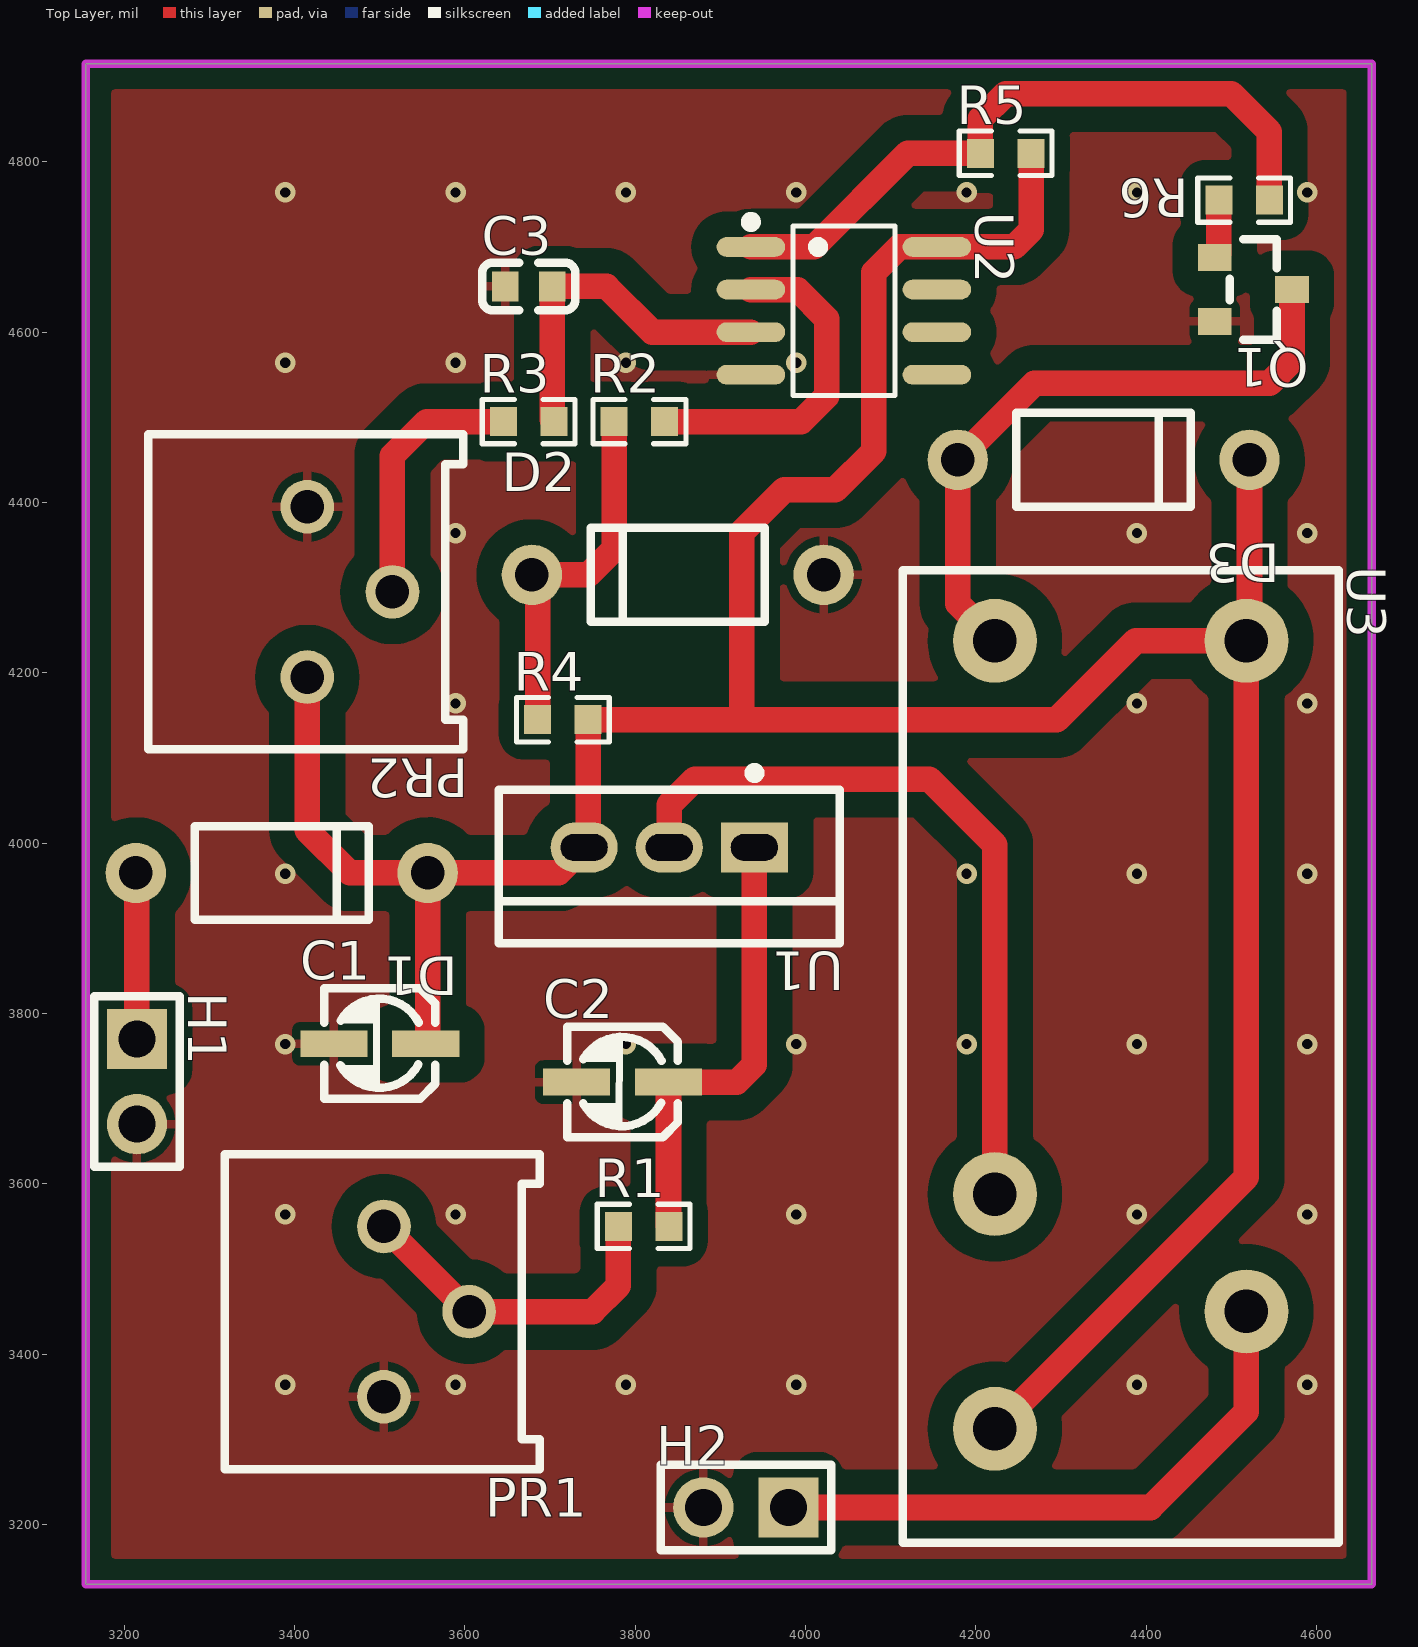
[diagram p0: Top Layer view]
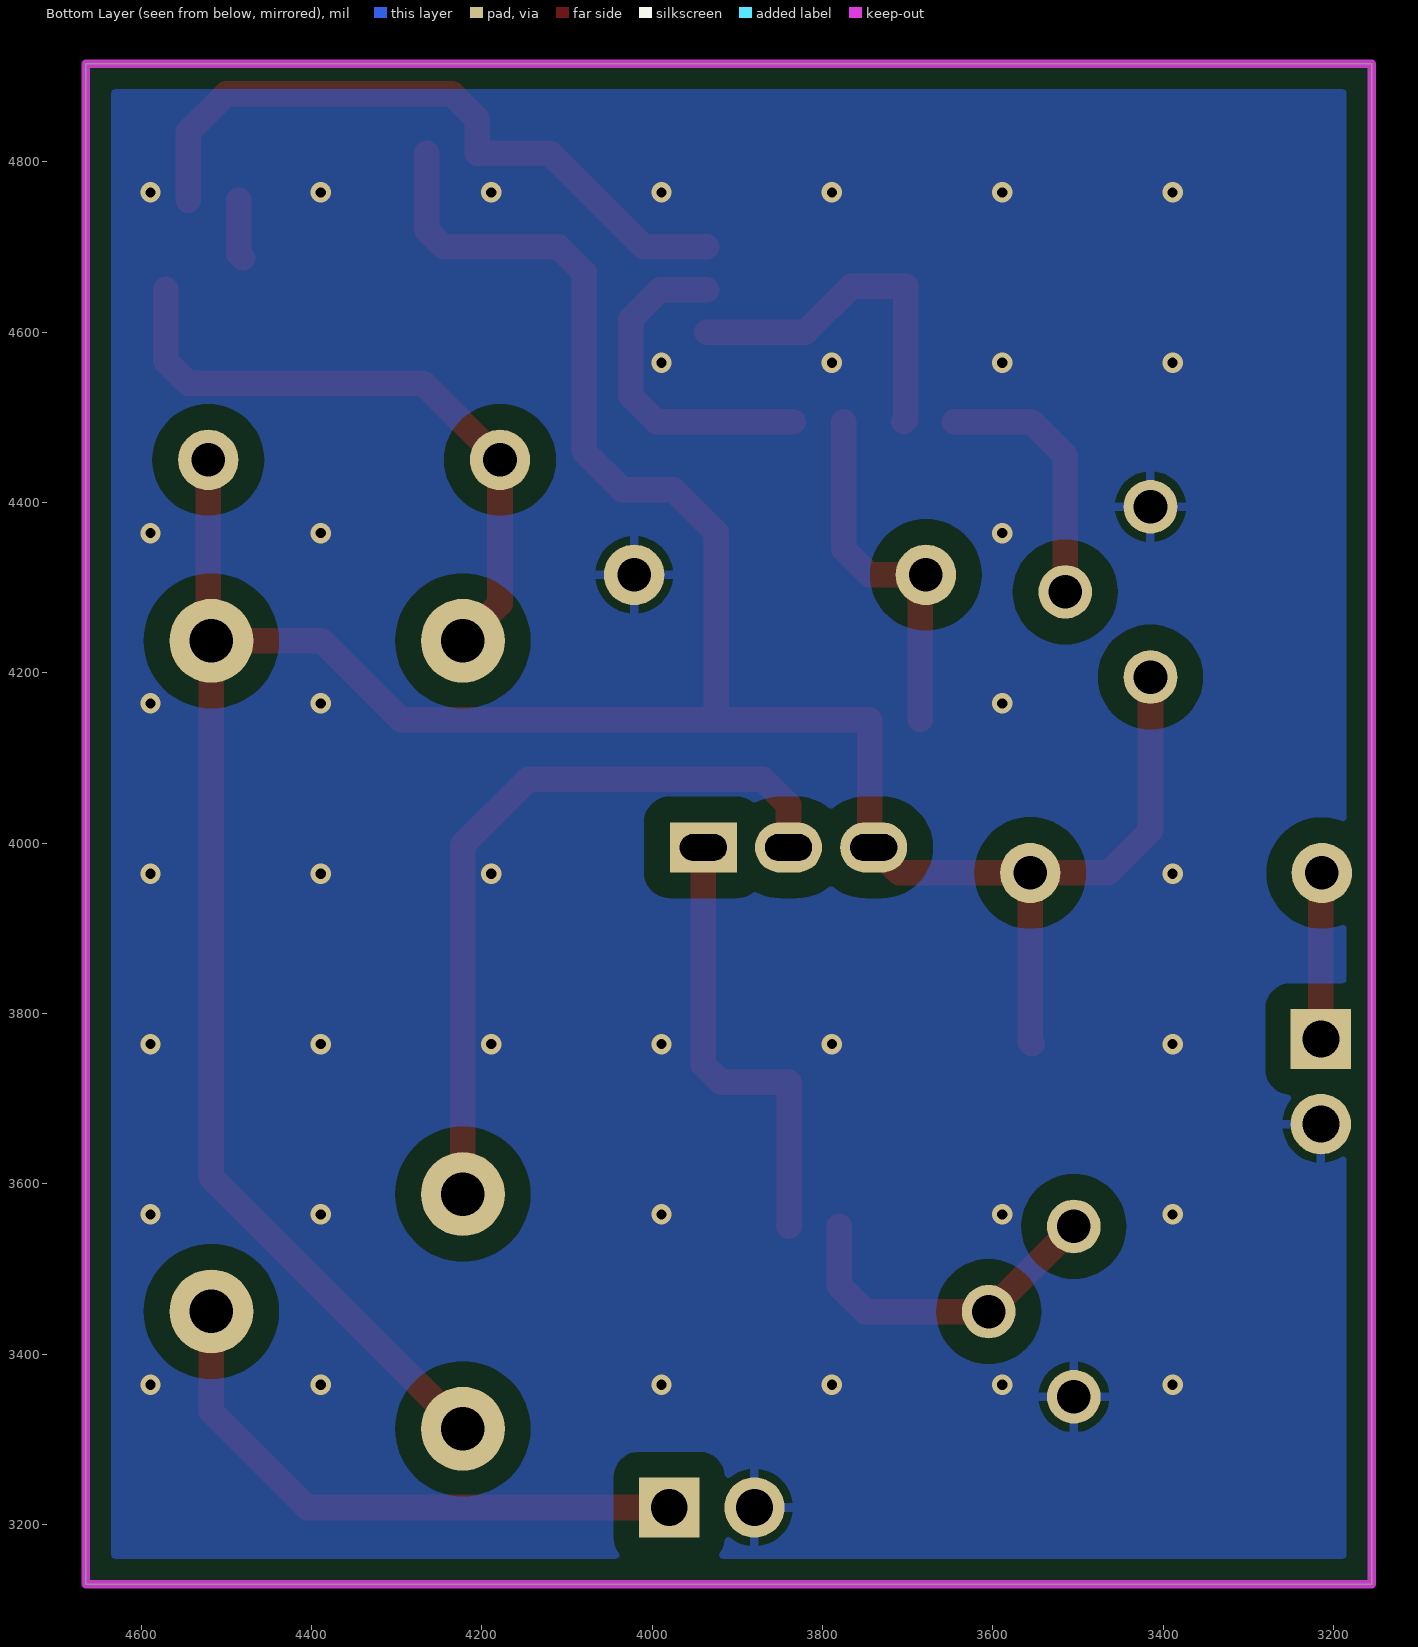
[diagram p1: Bottom Layer view, seen from below]
# Altium PCB MISC52117.pcbdoc
Units mil, origin at the board's own origin, x right, y up, seen from the top; angles counter-clockwise.
Board outline 1510 x 1785 mil, 2 copper layers (Top Layer, Bottom Layer), stack 62.206 mil thick; 20 components, 14 nets, 53 pads, 38 vias.

## Layer stack, top to bottom
Top Solder Mask Layer: solder mask 0.394, Dk 3.3
Top Layer: signal copper 1.379
Dielectric1: surface 59.449, FR4, Dk 4.5
Bottom Layer: signal copper 1.378
Bottom Solder Mask Layer: solder mask 0.394, Dk 3.3

## Board outline
3155,4915 3155,3130 4665,3130 4665,4915

## Design rules (kind name [scope] priority, off if disabled: settings)
BoardOutlineClearance copperThickness2oz_1 [All] p2 off: genericclearance=7.99 ignorepadtopadclearanceinfootprint=FALSE except(0: Arc-SplitContinuation Track-SplitContinuation SMDPad-SplitContinuation THPad-SplitContinuation Via-SplitContinuation Fill-SplitContinuation Region-SplitContinuation Poly-SplitContinuation Text-SplitContinuation Hole-SplitContinuation; 5.98: Arc-CutoutEdge Track-CutoutEdge SMDPad-CutoutEdge THPad-CutoutEdge Via-CutoutEdge Text-CutoutEdge; 6.89: Hole-OutlineEdge Hole-CutoutEdge; 11.81: Arc-OutlineEdge Track-OutlineEdge SMDPad-OutlineEdge THPad-OutlineEdge Via-OutlineEdge Fill-OutlineEdge Region-OutlineEdge Text-OutlineEdge Fill-CutoutEdge Region-CutoutEdge; 30: Poly-OutlineEdge Poly-CutoutEdge)
BoardOutlineClearance Plane_innerPlane_1 [All] p4 off: genericclearance=4.02 ignorepadtopadclearanceinfootprint=FALSE except(0: Arc-SplitContinuation Track-SplitContinuation SMDPad-SplitContinuation THPad-SplitContinuation Via-SplitContinuation Fill-SplitContinuation Region-SplitContinuation Poly-SplitContinuation Text-SplitContinuation Hole-SplitContinuation; 5.98: Arc-CutoutEdge Track-CutoutEdge SMDPad-CutoutEdge THPad-CutoutEdge Via-CutoutEdge Text-CutoutEdge; 6.89: Hole-OutlineEdge Hole-CutoutEdge; 10: Poly-OutlineEdge Poly-CutoutEdge; 11.81: Arc-OutlineEdge Track-OutlineEdge SMDPad-OutlineEdge THPad-OutlineEdge Via-OutlineEdge Fill-OutlineEdge Region-OutlineEdge Text-OutlineEdge Fill-CutoutEdge Region-CutoutEdge)
BoardOutlineClearance Copper_copperRegion_1 [All] p6 off: genericclearance=4.02 ignorepadtopadclearanceinfootprint=FALSE except(0: Arc-SplitContinuation Track-SplitContinuation SMDPad-SplitContinuation THPad-SplitContinuation Via-SplitContinuation Fill-SplitContinuation Region-SplitContinuation Poly-SplitContinuation Text-SplitContinuation Hole-SplitContinuation; 5.98: Arc-CutoutEdge Track-CutoutEdge SMDPad-CutoutEdge THPad-CutoutEdge Via-CutoutEdge Text-CutoutEdge; 6.89: Hole-OutlineEdge Hole-CutoutEdge; 11.81: Arc-OutlineEdge Track-OutlineEdge SMDPad-OutlineEdge THPad-OutlineEdge Via-OutlineEdge Fill-OutlineEdge Region-OutlineEdge Text-OutlineEdge Fill-CutoutEdge Region-CutoutEdge; 30: Poly-OutlineEdge Poly-CutoutEdge)
BoardOutlineClearance copperThickness1oz_1 [All] p8: genericclearance=4.02 ignorepadtopadclearanceinfootprint=FALSE except(0: Arc-SplitContinuation Track-SplitContinuation SMDPad-SplitContinuation THPad-SplitContinuation Via-SplitContinuation Fill-SplitContinuation Region-SplitContinuation Poly-SplitContinuation Text-SplitContinuation Hole-SplitContinuation; 5.98: Arc-CutoutEdge Track-CutoutEdge SMDPad-CutoutEdge THPad-CutoutEdge Via-CutoutEdge Text-CutoutEdge; 6.89: Hole-OutlineEdge Hole-CutoutEdge; 11.81: Arc-OutlineEdge Track-OutlineEdge SMDPad-OutlineEdge THPad-OutlineEdge Via-OutlineEdge Fill-OutlineEdge Region-OutlineEdge Text-OutlineEdge Fill-CutoutEdge Region-CutoutEdge; 30: Poly-OutlineEdge Poly-CutoutEdge)
Clearance copperThickness2oz [All] p1 off: gap=7.99 ignorepadtopadclearanceinfootprint=FALSE except(5.98: SMDPad-Track SMDPad-SMDPad THPad-Track SMDPad-THPad THPad-THPad Track-Via SMDPad-Via THPad-Via Via-Via Fill-SMDPad Region-SMDPad Fill-THPad Region-THPad Fill-Via Region-Via Fill-Fill Fill-Region Region-Region Arc-Track Arc-SMDPad Arc-THPad Arc-Via Fill-Arc Region-Arc Arc-Arc Text-Track SMDPad-Text Text-THPad Text-Via Fill-Text Region-Text Arc-Text Text-Text; 6.89: Hole-Track Hole-SMDPad Hole-THPad Hole-Via Fill-Hole Region-Hole Hole-Arc Hole-Text; 11.81: Fill-Track Region-Track; 30: Poly-Track Poly-SMDPad Poly-THPad Poly-Via Poly-Fill Poly-Region Poly-Poly Poly-Arc Poly-Text Poly-Hole)
Clearance Plane_innerPlane [All] p3 off: gap=4.02 ignorepadtopadclearanceinfootprint=FALSE except(5.98: SMDPad-Track SMDPad-SMDPad THPad-Track SMDPad-THPad THPad-THPad Track-Via SMDPad-Via THPad-Via Via-Via Fill-SMDPad Region-SMDPad Fill-THPad Region-THPad Fill-Via Region-Via Fill-Fill Fill-Region Region-Region Arc-Track Arc-SMDPad Arc-THPad Arc-Via Fill-Arc Region-Arc Arc-Arc Text-Track SMDPad-Text Text-THPad Text-Via Fill-Text Region-Text Arc-Text Text-Text; 6.89: Hole-Track Hole-SMDPad Hole-THPad Hole-Via Fill-Hole Region-Hole Hole-Arc Hole-Text; 10: Poly-Track Poly-SMDPad Poly-THPad Poly-Via Poly-Fill Poly-Region Poly-Poly Poly-Arc Poly-Text Poly-Hole; 11.81: Fill-Track Region-Track)
Clearance Copper_copperRegion [All] p5 off: gap=4.02 ignorepadtopadclearanceinfootprint=FALSE except(5.98: SMDPad-Track SMDPad-SMDPad THPad-Track SMDPad-THPad THPad-THPad Track-Via SMDPad-Via THPad-Via Via-Via Fill-SMDPad Region-SMDPad Fill-THPad Region-THPad Fill-Via Region-Via Fill-Fill Fill-Region Region-Region Arc-Track Arc-SMDPad Arc-THPad Arc-Via Fill-Arc Region-Arc Arc-Arc Text-Track SMDPad-Text Text-THPad Text-Via Fill-Text Region-Text Arc-Text Text-Text; 6.89: Hole-Track Hole-SMDPad Hole-THPad Hole-Via Fill-Hole Region-Hole Hole-Arc Hole-Text; 11.81: Fill-Track Region-Track; 30: Poly-Track Poly-SMDPad Poly-THPad Poly-Via Poly-Fill Poly-Region Poly-Poly Poly-Arc Poly-Text Poly-Hole)
Clearance copperThickness1oz [All] p7: gap=4.02 ignorepadtopadclearanceinfootprint=FALSE except(5.98: SMDPad-Track SMDPad-SMDPad THPad-Track SMDPad-THPad THPad-THPad Track-Via SMDPad-Via THPad-Via Via-Via Fill-SMDPad Region-SMDPad Fill-THPad Region-THPad Fill-Via Region-Via Fill-Fill Fill-Region Region-Region Arc-Track Arc-SMDPad Arc-THPad Arc-Via Fill-Arc Region-Arc Arc-Arc Text-Track SMDPad-Text Text-THPad Text-Via Fill-Text Region-Text Arc-Text Text-Text; 6.89: Hole-Track Hole-SMDPad Hole-THPad Hole-Via Fill-Hole Region-Hole Hole-Arc Hole-Text; 11.81: Fill-Track Region-Track; 30: Poly-Track Poly-SMDPad Poly-THPad Poly-Via Poly-Fill Poly-Region Poly-Poly Poly-Arc Poly-Text Poly-Hole)
DiffPairsRouting differentialPair [All] p1: maxlimit=6 minlimit=6 mostfreqgap=6 toplayer_minwidth=5 toplayer_prefwidth=10 toplayer_maxwidth=100 toplayer_mingap=6 toplayer_prefgap=6 toplayer_maxgap=6 bottomlayer_minwidth=5 bottomlayer_prefwidth=10 bottomlayer_maxwidth=100 bottomlayer_mingap=6 bottomlayer_prefgap=6 bottomlayer_maxgap=6 maxuncoupledlength=10
HoleToHoleClearance otherClearance [All] p1: gap=11.81 allowstackedmicrovias=TRUE
Length netLength [All] p1: minlimit=0 maxlimit=0
PasteMaskExpansion pasteMaskExpansion [All] p1: expansion=0
PlaneConnect innerPlane [All] p1: planeconnectstyle=Relief reliefexpansion=20 reliefentries=4 reliefconductorwidth=10 reliefairgap=10
PolygonConnect copperRegion [All] p1: connectstyle=Relief reliefconductorwidth=10 reliefentries=4 polygonreliefangle="90 Angle" airgapwidth=10 via.connectstyle=Relief via.reliefconductorwidth=10 via.reliefentries=4 via.polygonreliefangle="90 Angle" via.airgapwidth=10
RoutingVias viaSize [All] p1: holewidth=12.01 width=24.02 viastyle="Through Hole" minholewidth=11.81 minwidth=19.68 maxholewidth=248.03 maxwidth=393.7
SolderMaskExpansion solderMaskExpansion [IsVia] p1: expansion=-1000 istentingtop=TRUE
SolderMaskExpansion solderMaskExpansion [All] p2: expansion=2.01 istentingtop=FALSE
Width copperThickness2oz_2 [All] p1 off: maxlimit=100 minlimit=8 preferedwidth=10
Width copperThickness1oz_2 [All] p2: maxlimit=100 minlimit=5 preferedwidth=10

## Components (designator, comment, footprint, x,y, rotation, side; value= is the part's Value field where it differs from the comment)
C1 "1uF" C_Ele_SMD_3x5.4mm 3500,3765 r0 top
C2 "10uF" C_Ele_SMD_3x5.4mm 3785,3720 r0 top
C3 "100nF" C0603 3675.01,4653.68 r180 top
D1 "" DO_1N4007 3385,3965 r180 top
D2 "" DO_1N4007 3850,4315 r0 top
D3 "" DO_1N4007 4350,4450 r180 top
H1 "" HDR-TH_2P-P2.54-V-M-1 3215,3720.1 r270 top
H2 "" HDR-TH_2P-P2.54-V-M-1 3930,3220 r180 top
PR1 "10K" R_3386P 3505,3450 r180 top
PR2 "200K" R_3386P 3415,4295 r180 top
Q1 "" S8050_SOT-23 4525.85,4655.05 r180 top
R1 "240" R0603 3810,3550 r0 top
R2 "4.7K" R0603 3805,4495 r0 top
R3 "4.7K" R0603 3675,4495 r0 top
R4 "4.7K" R0603 3715,4145 r0 top
R5 "10K" R0603 4235,4810 r0 top
R6 "4.7K" R0603 4515,4755 r0 top
U1 "LM317T" TO-220-3_L10.2-W4.6-P2.54-L 3840,3995 r180 top
U2 "LM393DG4" SOIC-8_L4.9-W3.9-P1.27-LS6.0-BL 4045,4625 r270 top
U3 "G2R-1 继电器座" RELAY-TH_G2R-1_C9900014679 4370,3775 r270 top

## Footprints (in the part's own frame and the unit in brackets; to place one, negate y for a bottom-side part, rotate by r counter-clockwise, add the part's x,y. Pads: shape width x height; smd on the part's side, far side on the other; paste and mask are expansions set on the pad)
C0603 [mm]
  rect 0.8x0.9 smd: 1(-0.7,0) 2(0.7,0)
  silkscreen extent -1.39,-0.71 1.39,0.71
C_Ele_SMD_3x5.4mm [mil]
  rect 78.7x31.5 smd paste+0 mask+2: 1(54.1,-0.55) 2(-53.7,-0.55)
  silkscreen extent -65,-65 65,65
DO_1N4007 [mm]
  round 1.8 hole 1 paste+0 mask+0.051: 1(-4.35,0) 2(4.35,0)
  silkscreen extent -2.6,-1.4 2.6,1.4
HDR-TH_2P-P2.54-V-M-1 [mm]
  rect 1.8x1.8 hole 1.1: 1(-1.27,0)
  round 1.8 hole 1.1: 2(1.27,0)
  silkscreen extent -2.54,-1.27 2.54,1.27
R0603 [mil]
  rect 31.75x34.02 smd paste-3937.01 mask+2: 1(-29.66,0) 2(29.66,0)
  silkscreen extent -55,-26 55,26
R_3386P [mil]
  round 63 hole 39.4 paste+0 mask+2: 1(0,-100) 2(-100,0) 3(0,100)
  silkscreen extent -183,-185 187,185
RELAY-TH_G2R-1_C9900014679 [mm]
  round 2.5 hole 1.3 paste+0 mask+0.05: 1(-11.75,-3.75) 2(4.75,-3.75) 3(11.75,-3.75) 4(8.25,3.75) 5(-11.75,3.75)
  silkscreen extent -13.85,-6.5 15.15,6.5
S8050_SOT-23 [mm]
  rect 1x0.8 smd paste+0 mask+0.051: 1(1.15,-0.823) 2(1.15,1.077) 3(-1.15,0.127)
  silkscreen extent -0.7,-1.37 0.7,1.63
SOIC-8_L4.9-W3.9-P1.27-LS6.0-BL [mm]
  oval 0.588x2.045 smd: 1(-1.905,-2.772) 2(-0.635,-2.772) 3(0.635,-2.772) 4(1.905,-2.772) 5(1.905,2.772) 6(0.635,2.772) 7(-0.635,2.772) 8(-1.905,2.772)
  silkscreen extent -2.8,-2.92 2.53,1.52
TO-220-3_L10.2-W4.6-P2.54-L [mm]
  rect 2x1.5 hole 0.8 slot 1.4 at 0 deg: 1(-2.54,0)
  oval 2x1.5 hole 0.8 slot 1.4 at 0 deg: 2(0,0) 3(2.54,0)
  silkscreen extent -5.08,-2.37 5.08,2.86

## Via types
v1: diameter 24.02, hole 12, Top Layer to Bottom Layer, 38 vias

## Nets (pads, with @x,y where several pads share a name; then routed paths per layer and width w, separated by ;. In a path a pad name is that pad's centre, name@x,y a point inside that pad or via, vN(x,y) a via of type N, cw(c..) or ccw(c..) an arc to the next point about the centre after c; other vN are vias at no path point)
$1N158: D1.2 H1.1 | length 195.4
  Top Layer w30: D1.2 3215,3963.74 H1.1
$1N520: PR1.1 PR1.2 R1.1 | length 399
  Top Layer w30: PR1.1 PR1.2 3750,3450 3780.34,3480.34 R1.1
$1N588: C2.1 R1.2 U1.1 | length 534.1
  Top Layer w30: R1.2 3839.1,3550.56 C2.1 3919.45,3719.45 3940,3740 U1.1
$1N803: R2.2 U2.2 | length 396.7
  Top Layer w30: R2.2 3995,4495 4025,4525 4025,4615.56 3990.56,4650 U2.2
$1N937: C3.1 R3.2 U2.3 | length 415.1
  Top Layer w30: R3.2 3702.57,4497.09 C3.1 3766.32,4653.68 3820,4600 U2.3
$1N975: PR2.2 R3.1 | length 306.9
  Top Layer w30: PR2.2 3515,4455 3555,4495 R3.1
$1N1107: D2.1 R2.1 R4.1 | length 431.6
  Top Layer w30: R4.1 3685.34,4308.4 D2.1 3745,4315 3775.34,4345.34 R2.1
$1N1293: R5.1 R6.2 U2.1 | length 805.8
  Top Layer w30: U2.1 4010,4700 4120,4810 R5.1 4205.34,4850.34 4235,4880 4500,4880 4544.66,4835.34 R6.2
$1N1350: Q1.1 R6.1 | length 69.5
  Top Layer w30: Q1.1 4485.34,4692.21 R6.1
$1N1577: D3.2 Q1.3 U3.1 | length 754.9
  Top Layer w30: U3.1 4178.74,4281.22 D3.2 4268.74,4540 4545,4540 4571.13,4566.13 Q1.3
$1N1650: H2.1 U3.4 | length 701.9
  Top Layer w30: H2.1 4405,3220 4517.64,3332.64 U3.4
EOUT: U1.2 U3.2 | length 886.7
  Top Layer w30: U1.2 3840,4045 3870,4075 4145.4,4075 4222.36,3998.04 U3.2
EVCC: C1.1 D1.1 D3.1 PR2.3 R4.2 R5.2 U1.3 U2.8 U3.3 U3.5 | length 3884.4
  Top Layer w30: PR2.3 3415,4015 3465,3965 D1.1 ; C1.1 3556.26,3766.61 D1.1 ; U3.3 4517.64,3607.67 U3.5 ; R5.2 4265,4809.66 4265,4720 4245,4700 U2.8 4110,4700 4080,4670 4080,4460 4035,4415 3975,4415 3925,4365 3925,4145 ; D3.1 4521.26,4241.22 U3.5 ; D1.1 3709.99,3965 U1.3 3744.66,3999.67 R4.2 3925,4145 ; 3925,4145 4295,4145 4387.6,4237.6 U3.5
GND: C1.2 C2.2 C3.2 D2.2 H1.2 H2.2 PR1.3 PR2.1 Q1.2 U2.4
  other v1: 3389.1,3364.1 3589.1,3364.1 3789.1,3364.1 3989.1,3364.1 4389.1,3364.1 4589.1,3364.1 3389.1,3564.1 3589.1,3564.1 3989.1,3564.1 4389.1,3564.1 4589.1,3564.1 3389.1,3764.1 3789.1,3764.1 3989.1,3764.1 4189.1,3764.1 4389.1,3764.1 4589.1,3764.1 3389.1,3964.1 4189.1,3964.1 4389.1,3964.1 4589.1,3964.1 3589.1,4164.1 4389.1,4164.1 4589.1,4164.1 3589.1,4364.1 4389.1,4364.1 4589.1,4364.1 3389.1,4564.1 3589.1,4564.1 3789.1,4564.1 3989.1,4564.1 3389.1,4764.1 3589.1,4764.1 3789.1,4764.1 3989.1,4764.1 4189.1,4764.1 4389.1,4764.1 4589.1,4764.1
pads on no net: U2.5 U2.6 U2.7

## Polygon pours and split planes (outlines as drawn)
GND on Top Layer (solid, remove dead copper, pour order 0): 3010,5030 3010,3020 4830,3020 4830,5030
GND on Bottom Layer (solid, remove dead copper, pour order 2): 3000,5020 3000,3000 4900,3000 4900,5020

## Keep-outs
Board Outline Layer:
  the board outline again, w10